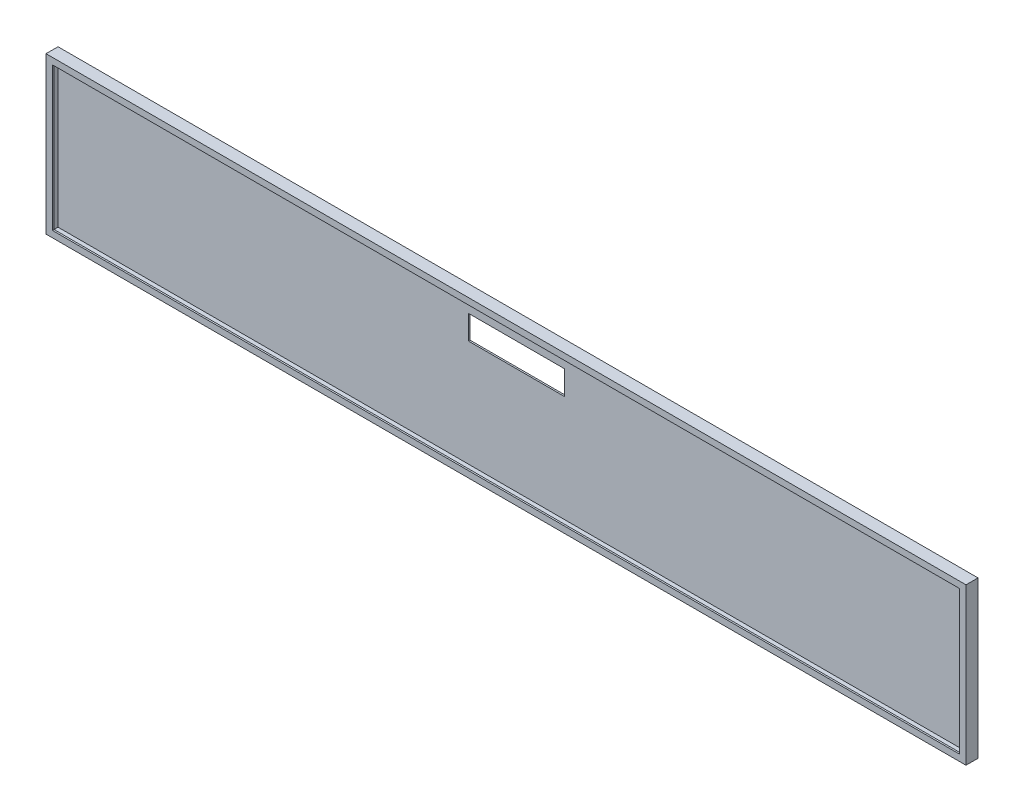
SolidWorks part; units mm, degrees
ref_plane "前视基准面" through (0, 0, 0) normal (0, 0, 1) x (1, 0, 0)
ref_plane "上视基准面" through (0, 0, 0) normal (0, 1, 0) x (1, 0, 0)
ref_plane "右视基准面" through (0, 0, 0) normal (1, 0, 0) x (0, 0, -1)
sketch "草图1" plane through (0, 0, 0) normal (0, 0, 1) x (1, 0, 0)
  line L1 (0, 0) -> (1148, 0)
  line L2 (0, 0) -> (0, 195)
  line L3 (0, 195) -> (1148, 195)
  line L4 (1148, 0) -> (1148, 195)
  dimension "D1" = 195
  dimension "D2" = 1148
extrude "凸台-拉伸1" add sketch "草图1" along normal blind 15
shell "抽壳1" thickness 2
sketch "草图2" plane through (0, 0, 15) normal (0, 0, 1) x (1, 0, 0)
  line L0 (8, 187) -> (8, 8)
  line L1 (0, 195) -> (1148, 195)
  line L2 (0, 195) -> (0, 0)
  line L3 (0, 0) -> (1148, 0)
  line L4 (1148, 195) -> (1148, 0)
  line L5 (8, 8) -> (1140, 8)
  line L6 (1140, 187) -> (1140, 8)
  line L7 (8, 187) -> (1140, 187)
  dimension "D1" = 8
extrude "凸台-拉伸2" add sketch "草图2" against normal blind 2
sketch "草图3" plane through (0, 0, 0) normal (0, 0, -1) x (-1, 0, 0)
  line L0 (-574, 195) -> (-574, -61.0578) construction
  line L1 (-1148, 195) -> (0, 195) construction
  line L3 (-634, 165) -> (-514, 165)
  line L4 (-634, 165) -> (-634, 135)
  line L5 (-634, 135) -> (-514, 135)
  line L6 (-514, 165) -> (-514, 135)
  dimension "D1" = 120
  dimension "D2" = 60
  dimension "D3" = 30
  dimension "D4" = 30
extrude "切除-拉伸1" cut sketch "草图3" against normal blind 10
